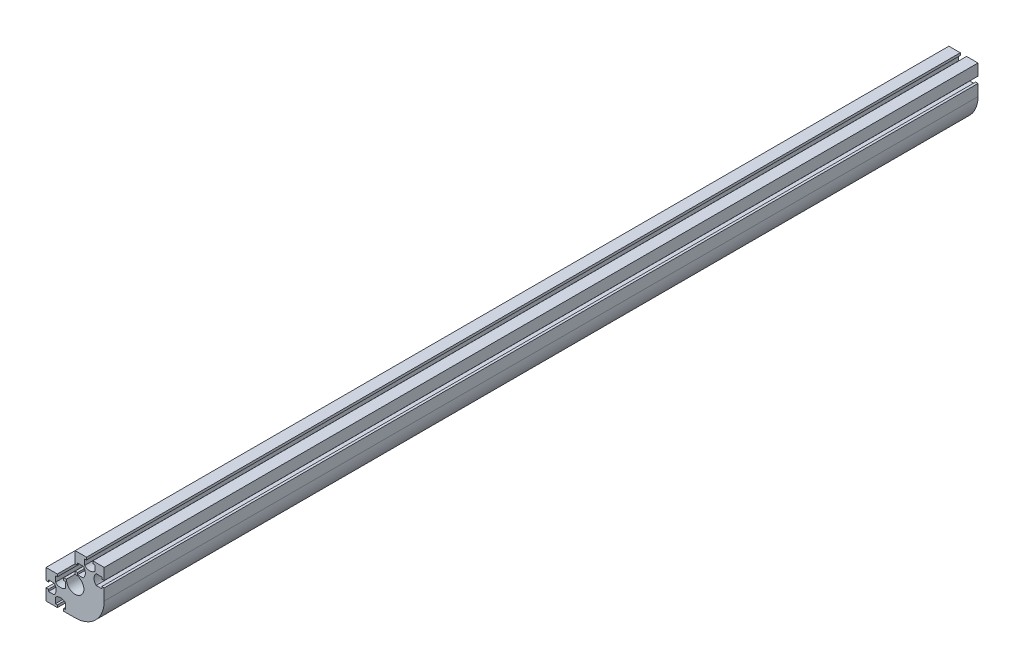
SolidWorks part; units mm, degrees
ref_plane "前视基准面" through (0, 0, 0) normal (0, 0, 1) x (1, 0, 0)
ref_plane "上视基准面" through (0, 0, 0) normal (0, 1, 0) x (1, 0, 0)
ref_plane "右视基准面" through (0, 0, 0) normal (1, 0, 0) x (0, 0, -1)
sketch "草图1" plane through (0, 0, 0) normal (0, 0, 1) x (1, 0, 0)
  line L0 (0, 9) -> (0, 11.75)
  line L1 (0, 30) -> (11.75, 30)
  line L2 (30, 30) -> (30, 18.25)
  line L4 (-30, 0) -> (-30, -11.75)
  line L5 (-30, -30) -> (-18.25, -30)
  line L6 (0, 0) -> (-35355.3391, 35355.3391) construction
  line L7 (-11.75, 0) -> (-11.75, -2.5)
  line L8 (-11.75, -2.5) -> (-9.75, -2.5)
  line L9 (-9.75, -2.5) -> (-9.75, -8.36)
  line L10 (-18.25, 0) -> (-18.25, -2.5)
  line L11 (-18.25, -2.5) -> (-20.25, -2.5)
  line L12 (-20.25, -2.5) -> (-20.25, -8.36)
  line L13 (-23.25, -15) -> (0, -15) construction
  line L14 (-30, 0) -> (-18.25, 0)
  line L15 (-11.75, 0) -> (-9, 0)
  line L16 (-11.75, -30) -> (-11.75, -27.5)
  line L17 (-11.75, -27.5) -> (-9.75, -27.5)
  line L18 (-9.75, -27.5) -> (-9.75, -21.64)
  line L19 (-18.25, -27.5) -> (-20.25, -27.5)
  line L20 (-20.25, -27.5) -> (-20.25, -21.64)
  line L21 (-18.25, -30) -> (-18.25, -27.5)
  line L22 (-11.75, -30) -> (0, -30)
  line L24 (-30, -11.75) -> (-27.5, -11.75)
  line L27 (-27.5, -11.75) -> (-27.5, -9.75)
  line L29 (-27.5, -9.75) -> (-21.64, -9.75)
  line L30 (-30, -18.25) -> (-30, -30)
  line L31 (-27.5, -20.25) -> (-21.64, -20.25)
  line L32 (-27.5, -18.25) -> (-27.5, -20.25)
  line L33 (-30, -18.25) -> (-27.5, -18.25)
  line L34 (2.5, 9.75) -> (8.36, 9.75)
  line L35 (2.5, 11.75) -> (2.5, 9.75)
  line L36 (0, 11.75) -> (2.5, 11.75)
  line L37 (0, 18.25) -> (2.5, 18.25)
  line L38 (2.5, 18.25) -> (2.5, 20.25)
  line L39 (2.5, 20.25) -> (8.36, 20.25)
  line L40 (27.5, 9.75) -> (21.64, 9.75)
  line L41 (27.5, 11.75) -> (27.5, 9.75)
  line L42 (30, 11.75) -> (27.5, 11.75)
  line L43 (30, 18.25) -> (27.5, 18.25)
  line L44 (27.5, 18.25) -> (27.5, 20.25)
  line L45 (27.5, 20.25) -> (21.64, 20.25)
  line L46 (20.25, 27.5) -> (20.25, 21.64)
  line L47 (18.25, 27.5) -> (20.25, 27.5)
  line L48 (18.25, 30) -> (18.25, 27.5)
  line L49 (11.75, 30) -> (11.75, 27.5)
  line L50 (11.75, 27.5) -> (9.75, 27.5)
  line L51 (9.75, 27.5) -> (9.75, 21.64)
  line L52 (0, 18.25) -> (0, 30)
  line L53 (18.25, 30) -> (30, 30)
  line L54 (30, 11.75) -> (30, 0)
  arc A0 (0, -30) -> (30, 0) centre (0, 0) ccw
  arc A1 (-9, 0) -> (0, 9) centre (0, 0) ccw
  arc A3 (-20.25, -8.36) -> (-9.75, -8.36) centre (-15, -3) ccw
  arc A4 (-20.25, -21.64) -> (-9.75, -21.64) centre (-15, -27) cw
  arc A6 (-21.64, -20.25) -> (-21.64, -9.75) centre (-27, -15) ccw
  arc A7 (8.36, 20.25) -> (8.36, 9.75) centre (3, 15) cw
  arc A8 (21.64, 20.25) -> (21.64, 9.75) centre (27, 15) ccw
  arc A9 (20.25, 21.64) -> (9.75, 21.64) centre (15, 27) cw
  dimension "D1" = 60
  dimension "D2" = 18
  dimension "D9" = 2.5
  dimension "D3" = 2.75
  dimension "D4" = 2.5
  dimension "D5" = 2
  dimension "D6" = 5.86
  dimension "D7" = 6.5
  dimension "D8" = 2
  dimension "D10" = 2
  dimension "D11" = 5.86
extrude "凸台-拉伸1" add sketch "草图1" along normal blind 900
